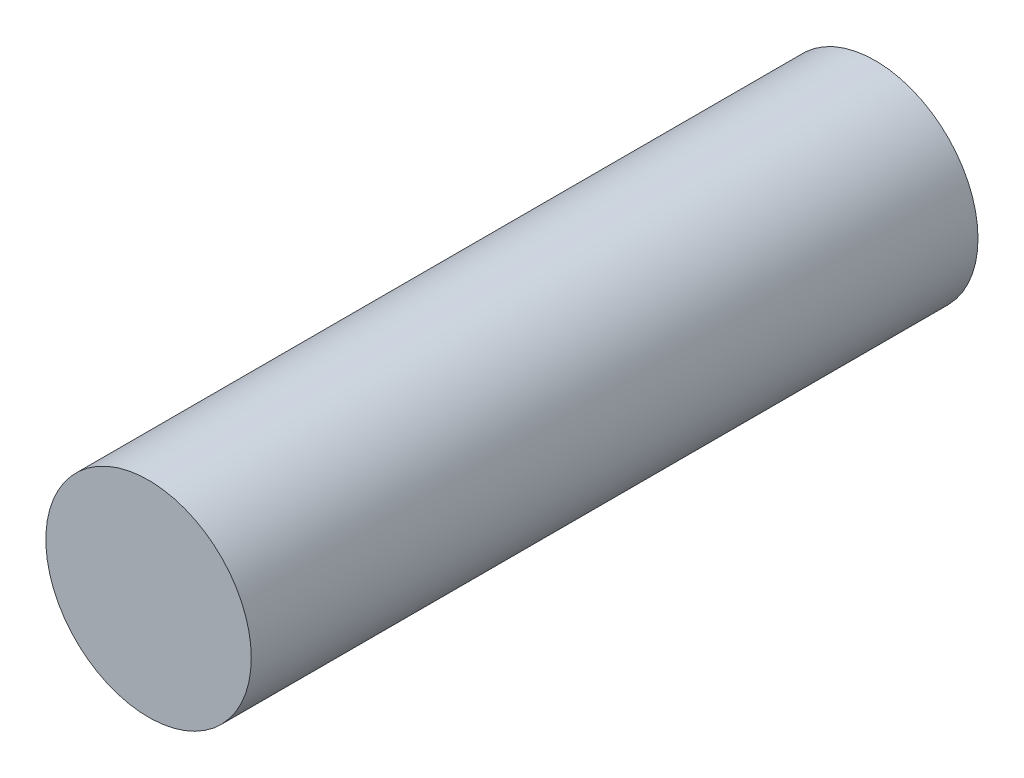
SolidWorks part; units mm, degrees
ref_plane "Front Plane" through (0, 0, 0) normal (0, 0, 1) x (1, 0, 0)
ref_plane "Top Plane" through (0, 0, 0) normal (0, 1, 0) x (1, 0, 0)
ref_plane "Right Plane" through (0, 0, 0) normal (1, 0, 0) x (0, 0, -1)
other "Configuration Table"
sketch "Sketch1" plane through (0, 0, 0) normal (0, 0, 1) x (1, 0, 0)
  circle A0 centre (-27.0657, 16.2887) radius 3.6746
extrude "Boss-Extrude1" add sketch "Sketch1" along normal mid plane 26
